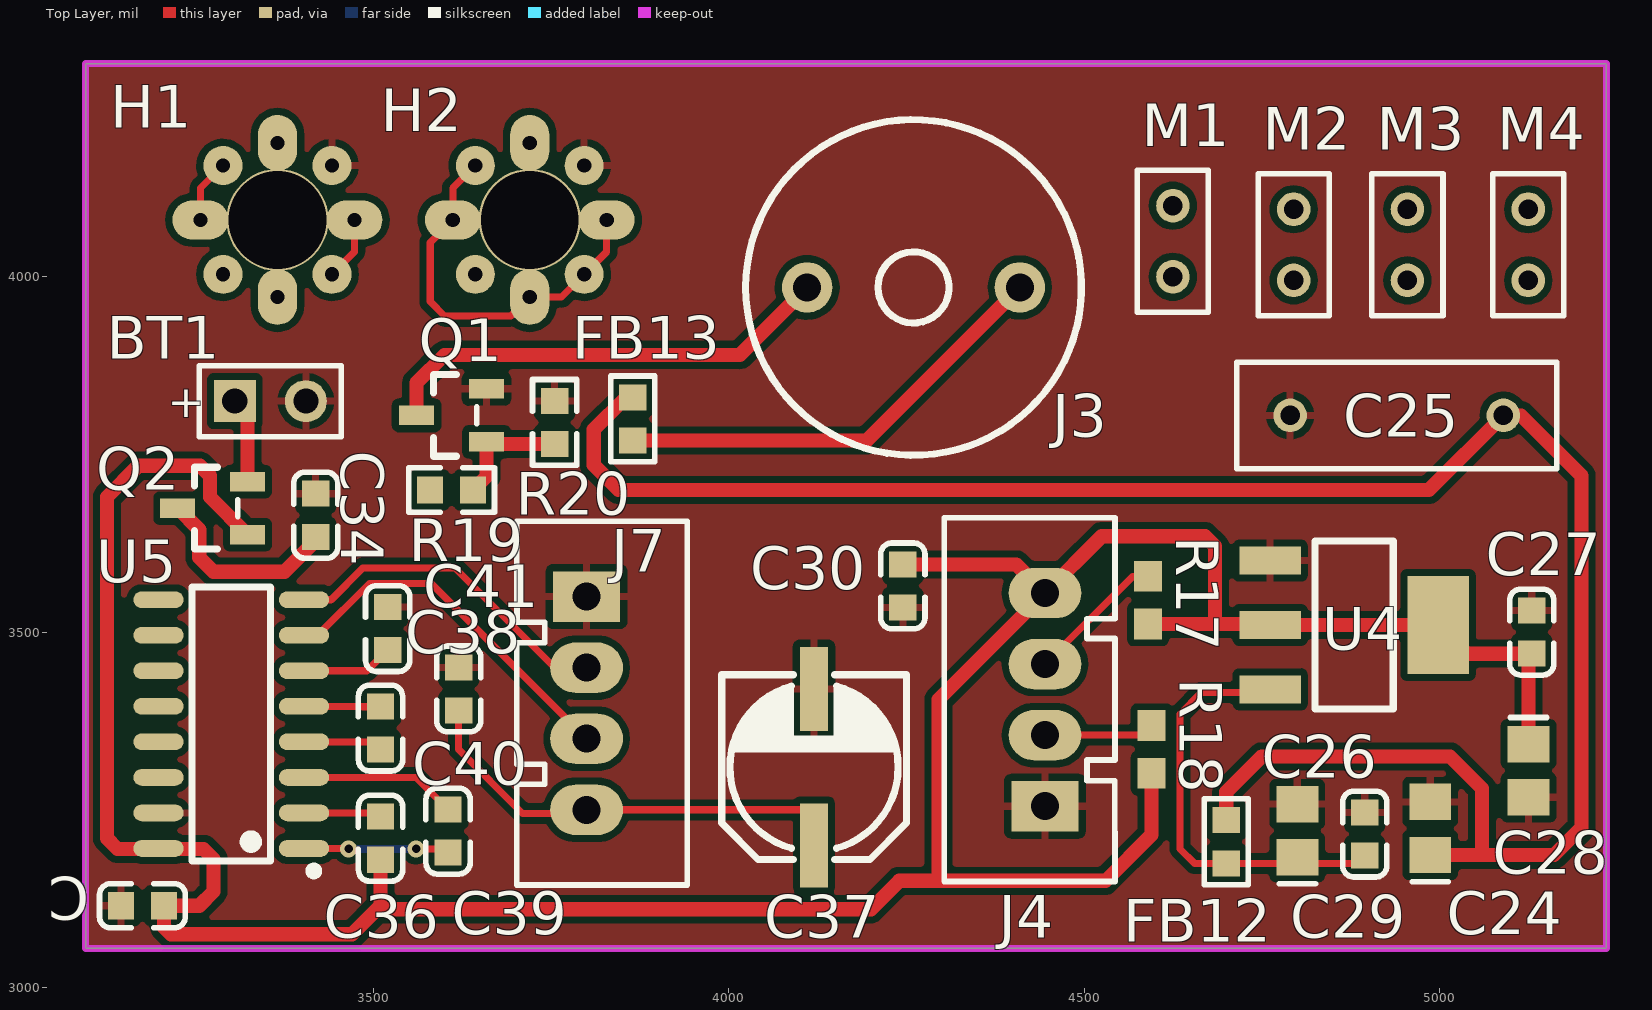
[diagram p0: Top Layer view]
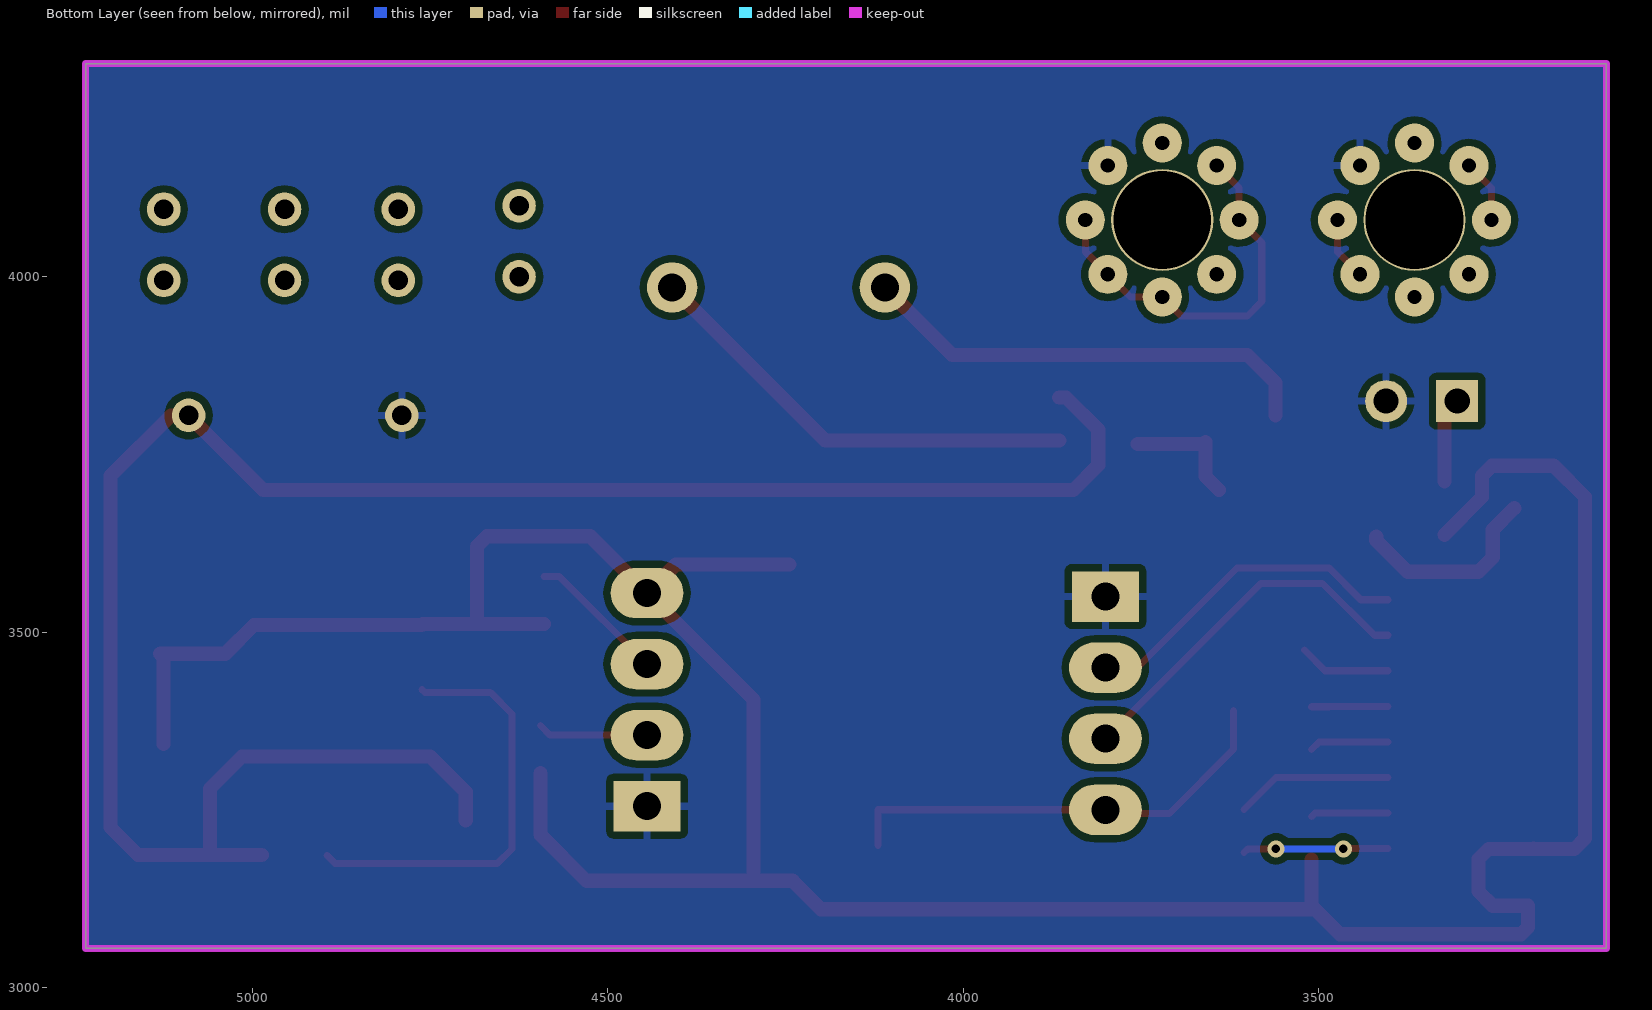
[diagram p1: Bottom Layer view, seen from below]
# Altium PCB MISC49890.pcbdoc
Units mil, origin at the board's own origin, x right, y up, seen from the top; angles counter-clockwise.
Board outline 2140 x 1245 mil, 2 copper layers (Top Layer, Bottom Layer); 35 components, 25 nets, 106 pads, 2 vias.

## Layer stack, top to bottom (the 12.6 mil dielectric is the usual default, probably not edited)
Top Solder Mask Layer: solder mask 0.4, Solder Resist, Dk 3.5
Top Layer: signal copper 1.4
Dielectric1: surface 12.6, FR-4, Dk 4.8
Bottom Layer: signal copper 1.4
Bottom Solder Mask Layer: solder mask 0.4, Solder Resist, Dk 3.5

## Board outline
3095,4300 3095,3055 5235,3055 5235,4300

## Design rules (kind name [scope] priority, off if disabled: settings)
BoardOutlineClearance Plane_PlaneConnect_1 [All] p2 off: genericclearance=10 ignorepadtopadclearanceinfootprint=FALSE except(0: Poly-OutlineEdge Poly-CutoutEdge Arc-SplitContinuation Track-SplitContinuation SMDPad-SplitContinuation THPad-SplitContinuation Via-SplitContinuation Fill-SplitContinuation Region-SplitContinuation Poly-SplitContinuation Text-SplitContinuation Hole-SplitContinuation; 10: Arc-OutlineEdge Track-OutlineEdge SMDPad-OutlineEdge THPad-OutlineEdge Via-OutlineEdge Fill-OutlineEdge Region-OutlineEdge Text-OutlineEdge Hole-OutlineEdge Arc-CutoutEdge Track-CutoutEdge SMDPad-CutoutEdge THPad-CutoutEdge Via-CutoutEdge Fill-CutoutEdge Region-CutoutEdge Text-CutoutEdge Hole-CutoutEdge)
BoardOutlineClearance Copper_PolygonConnect_1 [All] p4 off: genericclearance=10 ignorepadtopadclearanceinfootprint=FALSE except(0: Poly-OutlineEdge Poly-CutoutEdge Arc-SplitContinuation Track-SplitContinuation SMDPad-SplitContinuation THPad-SplitContinuation Via-SplitContinuation Fill-SplitContinuation Region-SplitContinuation Poly-SplitContinuation Text-SplitContinuation Hole-SplitContinuation; 10: Arc-OutlineEdge Track-OutlineEdge SMDPad-OutlineEdge THPad-OutlineEdge Via-OutlineEdge Fill-OutlineEdge Region-OutlineEdge Text-OutlineEdge Hole-OutlineEdge Arc-CutoutEdge Track-CutoutEdge SMDPad-CutoutEdge THPad-CutoutEdge Via-CutoutEdge Fill-CutoutEdge Region-CutoutEdge Text-CutoutEdge Hole-CutoutEdge)
BoardOutlineClearance Clearance_1 [All] p6: genericclearance=10 ignorepadtopadclearanceinfootprint=FALSE except(0: Arc-SplitContinuation Track-SplitContinuation SMDPad-SplitContinuation THPad-SplitContinuation Via-SplitContinuation Fill-SplitContinuation Region-SplitContinuation Poly-SplitContinuation Text-SplitContinuation Hole-SplitContinuation; 10: Arc-OutlineEdge Track-OutlineEdge SMDPad-OutlineEdge THPad-OutlineEdge Via-OutlineEdge Fill-OutlineEdge Region-OutlineEdge Poly-OutlineEdge Text-OutlineEdge Hole-OutlineEdge Arc-CutoutEdge Track-CutoutEdge SMDPad-CutoutEdge THPad-CutoutEdge Via-CutoutEdge Fill-CutoutEdge Region-CutoutEdge Poly-CutoutEdge Text-CutoutEdge Hole-CutoutEdge)
Clearance Plane_PlaneConnect [All] p1 off: gap=10 ignorepadtopadclearanceinfootprint=FALSE except(0: Hole-Track Hole-SMDPad Hole-THPad Hole-Via Fill-Hole Region-Hole Hole-Arc Hole-Text; 6: Poly-Track Poly-SMDPad Poly-THPad Poly-Via Poly-Fill Poly-Region Poly-Poly Poly-Arc Poly-Text Poly-Hole)
Clearance Copper_PolygonConnect [All] p3 off: gap=10 ignorepadtopadclearanceinfootprint=FALSE except(0: Hole-Track Hole-SMDPad Hole-THPad Hole-Via Fill-Hole Region-Hole Hole-Arc Hole-Text)
Clearance [All] p5: gap=10 ignorepadtopadclearanceinfootprint=FALSE except(0: Hole-Track Hole-SMDPad Hole-THPad Hole-Via Fill-Hole Region-Hole Hole-Arc Hole-Text)
DiffPairsRouting [All] p1: maxlimit=10 minlimit=10 mostfreqgap=10 toplayer_minwidth=15 toplayer_prefwidth=15 toplayer_maxwidth=15 toplayer_mingap=10 toplayer_prefgap=10 toplayer_maxgap=10 bottomlayer_minwidth=15 bottomlayer_prefwidth=15 bottomlayer_maxwidth=15 bottomlayer_mingap=10 bottomlayer_prefgap=10 bottomlayer_maxgap=10 maxuncoupledlength=500
HoleToHoleClearance otherClearance [All] p1: gap=11.8 allowstackedmicrovias=TRUE
Length netLength [All] p1: minlimit=0 maxlimit=0
PolygonConnect [All] p1: connectstyle=Relief reliefconductorwidth=10 reliefentries=4 polygonreliefangle="90 Angle" airgapwidth=10 via.connectstyle=Relief via.reliefconductorwidth=10 via.reliefentries=4 via.polygonreliefangle="90 Angle" via.airgapwidth=10
RoutingVias [All] p1: holewidth=28 width=50 viastyle="Through Hole" minholewidth=28 minwidth=50 maxholewidth=28 maxwidth=50
SolderMaskExpansion [All] p1: expansion=4 istentingtop=FALSE
Width [All] p1: maxlimit=90 minlimit=10 preferedwidth=10
2 further rules are at their usual default settings.

## Components (designator, comment, footprint, x,y, rotation, side; value= is the part's Value field where it differs from the comment)
BT1 "CR1200/NC" BAT-2 3355,3825 r0 top
C24 "" C0805 4987.13,3223.7 r90 top
C25 "" RAD-0.3 4940,3805 r0 top
C26 "" C0805 4800,3220.63 r90 top
C27 "Cap" 0603_C 5130,3500 r270 top
C28 "" C0805 5125.51,3305 r270 top
C29 "Cap" 0603_C 4895,3215.83 r270 top
C30 "Cap" 0603_C 4245,3565 r270 top
C34 "Cap" 0603_C 3418.78,3664.45 r270 top
C35 "Cap" 0603_C 3175,3115 r180 top
C36 "Cap" 0603_C 3510,3210 r270 top
C37 "Cap Pol1" CAP-SMD_BD6.3-L6.6-W6.6-FD 4120,3310 r90 top
C38 "Cap" 0603_C 3620,3420 r90 top
C39 "Cap" 0603_C 3605,3220 r90 top
C40 "Cap" 0603_C 3510,3365 r90 top
C41 "Cap" 0603_C 3520,3505 r270 top
FB12 "FB" 0603_L 4700,3205 r270 top
FB13 "FB" 0603_L 3865,3800 r270 top
H1 "H" HOLE-ZR 3365,4080 r0 top
H2 "H" HOLE-ZR 3720,4080 r0 top
J3 "BEEP" BUZ-TH_BD12.0-P7.60-D0.6-FD 4260,3985 r180 top
J4 "HEADER4X2.54MM" CN4$2F$DIP$2F$P2.54B 4445,3405 r270 top
J7 "HEADER4X2.54MM" CN4$2F$DIP$2F$P2.54B 3800,3400 r90 top
M1 "MARK" RAD-0.1 4625,4050 r90 top
M2 "MARK" RAD-0.1 4795,4045 r90 top
M3 "MARK" RAD-0.1 4955,4045 r90 top
M4 "MARK" RAD-0.1 5125,4045 r90 top
Q1 "S8050" SOT-23(SOT-23-3) 3610,3805 r0 top
Q2 "BAT54C" SOT-23(SOT-23-3) 3273.78,3674.45 r0 top
R17 "" J1-0603 4590,3545 r270 top
R18 "" J1-0603 4595,3335 r270 top
R19 "1K" 0603_R 3610,3700 r0 top
R20 "10K" 0603_R 3755,3795 r270 top
U4 "AMS1117-3.3V" SOT-223 4880,3510 r180 top
U5 "SP3232EEN" SOP-16_150MIL 3300,3370.59 r90 top

## Footprints (in the part's own frame and the unit in brackets; to place one, negate y for a bottom-side part, rotate by r counter-clockwise, add the part's x,y. Pads: shape width x height; smd on the part's side, far side on the other; paste and mask are expansions set on the pad)
0603_C [mm]
  rect 0.93x0.98 smd: 1(-0.77,0) 2(0.77,0)
  silkscreen extent -1.53,-0.79 1.54,0.79
0603_L [mm]
  rect 0.93x0.98 smd: 1(-0.77,0) 2(0.77,0)
  silkscreen extent -1.53,-0.79 1.54,0.79
0603_R [mm]
  rect 0.93x0.98 smd: 1(-0.77,0) 2(0.77,0)
  silkscreen extent -1.53,-0.79 1.54,0.79
BAT-2 [mm]
  rect 1.5x1.5 hole 0.9: 1(-1.27,0)
  round 1.5 hole 0.9: 2(1.27,0)
  silkscreen extent -2.54,-1.27 2.54,1.27
BUZ-TH_BD12.0-P7.60-D0.6-FD [mm]
  round 1.8 hole 1: 1(-3.8,0) 2(3.8,0)
  silkscreen extent -6,-6 6,6
C0805 [mm]
  rect 1.3x1.5 smd: 1(-0.95,0) 2(0.95,0)
  silkscreen extent -1.9,-0.65 -1.9,0.65
CAP-SMD_BD6.3-L6.6-W6.6-FD [mm]
  rect 3x1 smd: 1(-2.8,0) 2(2.8,0)
  silkscreen extent -3.3,-3.3 3.3,3.3
CN4$2F$DIP$2F$P2.54B [mm]
  rect 1.8x2.4 hole 1: 1(3.81,0)
  oval 1.8x2.6 hole 1: 2(1.27,0) 3(-1.27,0) 4(-3.81,0)
  silkscreen extent -6.5,-3.6 6.5,2.5
HOLE-ZR [mil]
  round 143.7 hole 137.8: 1(0,0)
  oval 55x78.74 / inner round 55 / far side round 55 hole 20: 2(0,108.27) 6(0,-108.27)
  round 55 hole 20: 3(-76.56,76.56) 5(-76.56,-76.56) 7(76.56,-76.56) 9(76.56,76.56)
  oval 78.74x55 / inner round 55 / far side round 55 hole 20: 4(-108.27,0) 8(108.27,0)
J1-0603 [mm]
  rect 1.1x1 smd: 1(-0.85,0) 2(0.85,0)
RAD-0.1 [mm]
  round 1.2 hole 0.7: 1(-1.27,0) 2(1.27,0)
  silkscreen extent -2.54,-1.27 2.54,1.27
RAD-0.3 [mm]
  round 1.2 hole 0.7: 1(-3.81,0) 2(3.81,0)
  silkscreen extent -5.71,-1.91 5.71,1.91
SOP-16_150MIL [mm]
  oval 0.6x1.8 smd: 1(-4.445,-2.6) 2(-3.175,-2.6) 3(-1.905,-2.6) 4(-0.635,-2.6) 5(0.635,-2.6) 6(1.905,-2.6) 7(3.175,-2.6) 8(4.445,-2.6) 9(4.445,2.6) 10(3.175,2.6) 11(1.905,2.6) 12(0.635,2.6) 13(-0.635,2.6) 14(-1.905,2.6) 15(-3.175,2.6) 16(-4.445,2.6)
  silkscreen extent -5.4,-3.1 4.9,1.4
SOT-23(SOT-23-3) [mm]
  rect 1.25x0.7 smd: 1(1.25,-0.95) 2(1.25,0.95) 3(-1.25,0)
  silkscreen extent -0.65,-1.46 0.9,1.46
SOT-223 [mm]
  rect 2.2x1 smd: 1(3,-2.3) 2(3,0) 3(3,2.3)
  rect 2.2x3.5 smd: 4(-3,0)
  silkscreen extent -1.4,-3 1.4,3

## Via types
v1: diameter 24, hole 12, Top Layer to Bottom Layer, 2 vias

## Nets (pads, with @x,y where several pads share a name; then routed paths per layer and width w, separated by ;. In a path a pad name is that pad's centre, name@x,y a point inside that pad or via, vN(x,y) a via of type N, cw(c..) or ccw(c..) an arc to the next point about the centre after c; other vN are vias at no path point)
$1N6: C26.1 C29.2 FB12.2 U4.3 | length 604.1
  Top Layer w10: U4.3 4757.44,3415 4665,3415 4635,3385 4635,3195 4655.32,3174.68 FB12.2 4884.17,3174.68 C29.2
$1N22: BT1.1 Q2.2 | length 120.6
  Top Layer w20: BT1.1 3322.99,3807.01 Q2.2
$1N24: H2.3 H2.4 H2.6 H2.7 H2.8 | length 556.6
  Top Layer w10: H2.3 3611.73,4124.85 H2.4 3580,4048.27 3580,3965 3600,3945 3693.27,3945 H2.6 3764.85,3971.73 H2.7 3828.27,4035.15 H2.8
$1N26: H1.1 H1.2 H1.3 H1.4 H1.6 H1.7 H1.8 | length 179.4
  Top Layer w10: H1.4 3256.73,4124.85 H1.3 ; H1.7 3473.27,4035.15 H1.8
$1N29: C40.2 U5.5 | length 108
  Top Layer w10: U5.5 3484.41,3395.59 3485,3395 3509.68,3395 C40.2
$1N30: C40.1 U5.4 | length 112.2
  Top Layer w10: U5.4 3499.09,3345.59 C40.1
$1N32: C41.2 U5.6 | length 129.7
  Top Layer w10: U5.6 3490.91,3445.59 C41.2
$1N35: C39.1 U5.1 | length 205.1
  Top Layer w10: U5.1 3464.41,3195.59 v1(3465,3195) ; v1(3560,3195) 3599.68,3195 C39.1
  Bottom Layer w10: v1(3465,3195) v1(3560,3195)
$1N36: C39.2 U5.3 | length 221.4
  Top Layer w10: U5.3 3559.72,3295.59 C39.2
$1N37: C36.1 U5.2 | length 109.8
  Top Layer w10: U5.2 3504.72,3245.59 C36.1
$1N764: J3.2 Q1.3 | length 651
  Top Layer w20: Q1.3 3560.79,3850.79 3600,3890 4015.39,3890 J3.2
$1N765: Q1.1 R19.2 R20.2 | length 172.4
  Top Layer w20: R19.2 3659.21,3718.9 Q1.1 3662.13,3764.68 R20.2
+5V: C24.1 C25.2 FB12.1 FB13.1 | length 2865.3
  Top Layer w20: FB13.1 3855.31,3830.31 3810,3785 3810,3735 3845,3700 4985,3700 C25.2 5115,3805 5200,3720 5200,3225 5161.3,3186.3 5064.13,3186.3 ; FB12.1 4700,3275 4750,3325 5015,3325 5060,3280 5060,3190.43 5064.13,3186.3 ; C24.1 5064.13,3186.3
BEEP: R19.1
GND: BT1.2 C24.2 C25.1 C26.2 C27.1 C28.2 C29.1 C30.2 C34.1 C35.2 C37.2 C38.2 C41.1 H1.9 H2.9 J4.1 J7.1 Q1.2 R20.1 U4.1 U5.15
MCU_RXD1: U5.9
MCU_TXD1: U5.10
RS232_RXD1: J7.2 U5.8 | length 474
  Top Layer w10: U5.8 3440.59,3545.59 3485,3590 3615,3590 3755,3450 J7.2
RS232_TXD1: J7.3 U5.7 | length 518.4
  Top Layer w10: U5.7 3421.46,3495.59 3494.5,3568.62 3581.38,3568.62 J7.3
SWCLK: J4.2 R18.1 | length 155.6
  Top Layer w10: J4.2 4581.54,3355 R18.1
SWDIO: J4.3 R17.1 | length 196.1
  Top Layer w10: J4.3 4568.46,3578.46 R17.1
TFT_12V: C37.1 C38.1 J7.4 | length 644.3
  Top Layer w10: C38.1 3620,3335 3710,3245 3795,3245 J7.4 4120,3250 C37.1
VBAT: C34.2 Q2.3 | length 277.6
  Top Layer w20: Q2.3 3255,3644.02 3255,3605 3275,3585 3375,3585 3418.78,3628.78 C34.2
VCC_3V3: C27.2 C28.1 C30.1 C35.1 C36.2 J4.4 Q2.1 R17.2 R18.2 U4.2 U4.4 U5.16 | length 4439
  Top Layer w20: Q2.1 3270,3690.04 3270,3720 3255.86,3734.14 3169.14,3734.14 3125,3690 3125,3210 3140,3195 3197.05,3195 U5.16 3198.23,3195 3260.86,3195 3275,3180.86 3275,3135 3255,3115 C35.1 3205.32,3084.68 3215,3075 3470,3075 3505,3110 ; C36.2 3510,3115 3505,3110 ; C30.1 4404.69,3595.32 J4.4 ; R17.2 4682.99,3511.54 ; R18.2 4595,3215 4530,3150 4295,3150 ; C28.1 5125.51,3465.2 C27.2 5038.43,3469.68 U4.4 U4.2 4760.35,3511.54 4682.99,3511.54 ; 3505,3110 4200,3110 4240,3150 4295,3150 ; 4295,3150 4295,3405 J4.4 ; J4.4 4525,3635 4670,3635 4684.14,3620.86 4684.14,3512.69 4682.99,3511.54
VCC_5V: FB13.2 J3.1 | length 633.8
  Top Layer w20: FB13.2 4194.29,3769.68 J3.1
pads on no net: H1.5 H2.1 H2.2 H2.5 M1.1 M1.2 M2.1 M2.2 M3.1 M3.2 M4.1 M4.2 U5.11 U5.12 U5.13 U5.14

## Polygon pours and split planes (outlines as drawn)
GND on Top Layer (solid, remove dead copper, pour order 0): 3015,4360 3015,3000 5255,3000 5255,4360
GND on Bottom Layer (solid, remove dead copper, pour order 2): 3000,4370 3000,3000 5315,3000 5315,4370

## Keep-outs
Board Outline Layer:
  the board outline again, w10